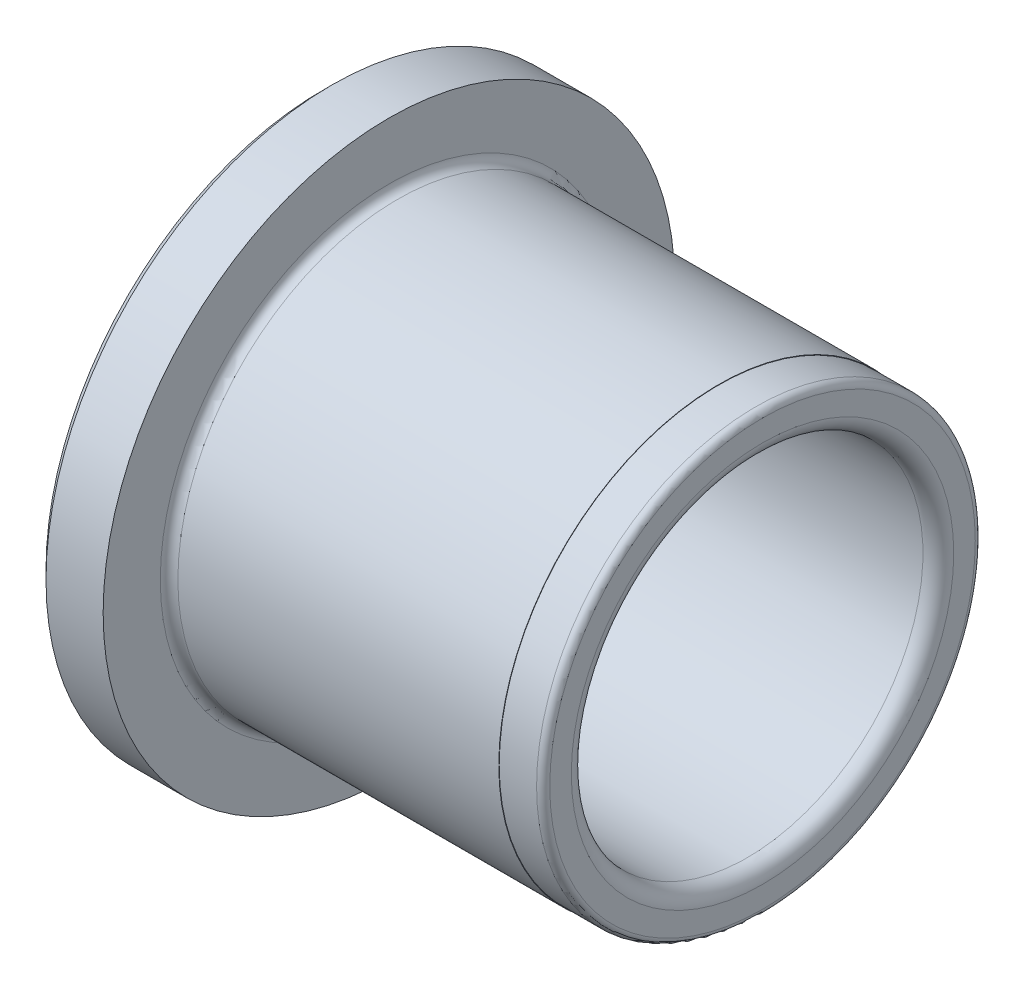
from build123d import *


with BuildPart() as part:
    # Sketch1 → Revolve1 (revolve)
    with BuildSketch(Plane.XY, mode=Mode.PRIVATE) as revolve1_sk:
        with BuildLine():
            Line((0, 12.6), (0, 9.116350684))
            ThreePointArc((0, 9.116350684), (0.16376889, 8.666399357), (0.578446276, 8.426985257))
            Line((0.578446276, 8.426985257), (3, 8))
            Line((3, 8), (19.3, 8))
            ThreePointArc((19.3, 8), (19.794974747, 8.205025253), (20, 8.7))
            Line((20, 8.7), (20, 9.68))
            ThreePointArc((20, 9.68), (19.912132034, 9.892132034), (19.7, 9.98))
            Line((19.7, 9.98), (18, 9.98))
            Line((18, 9.98), (18, 10))
            Line((18, 10), (3.4, 10))
            ThreePointArc((3.4, 10), (3.117157288, 10.117157288), (3, 10.4))
            Line((3, 10.4), (3, 13))
            Line((3, 13), (0.4, 13))
            Line((0.4, 13), (0, 12.6))
        make_face()
    revolve(revolve1_sk.sketch.rotate(Axis((20, 0, 0), (-1, 0, 0)), 270), axis=Axis((20, 0, 0), (-1, 0, 0)))


solid = part.part
